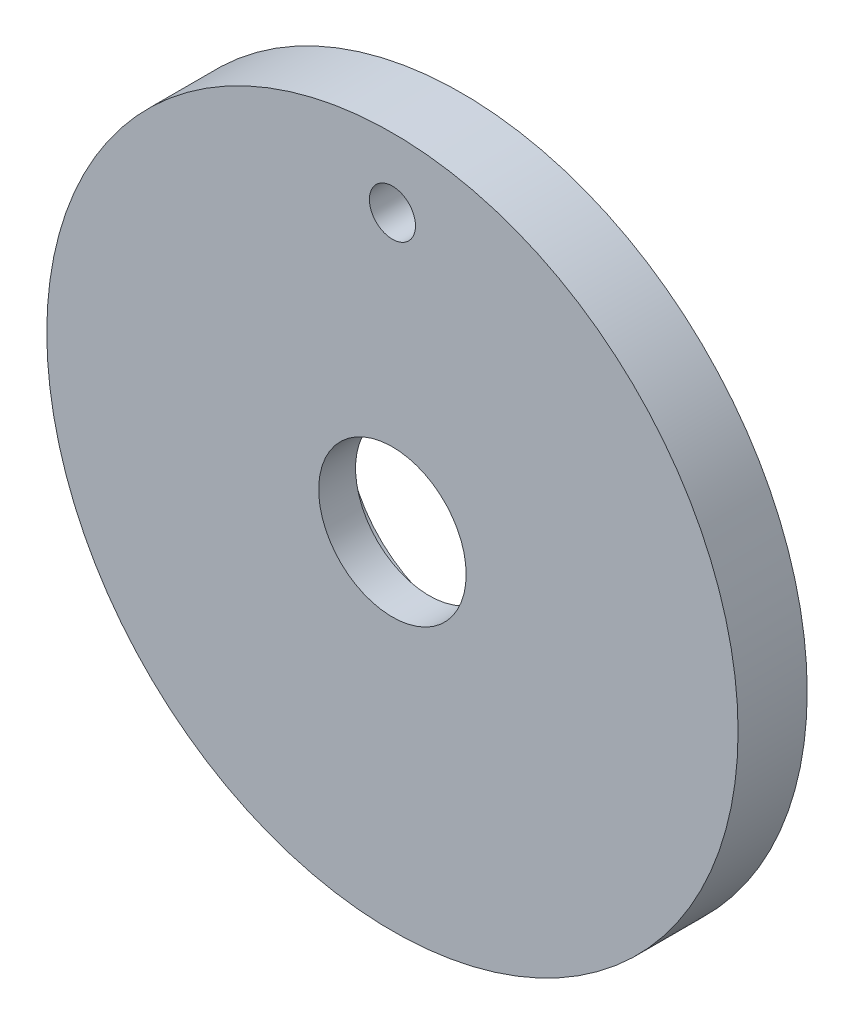
SolidWorks part; units mm, degrees
material "AISI 1045 钢，冷拔"
ref_plane "前视基准面" through (0, 0, 0) normal (0, 0, 1) x (1, 0, 0)
ref_plane "上视基准面" through (0, 0, 0) normal (0, 1, 0) x (1, 0, 0)
ref_plane "右视基准面" through (0, 0, 0) normal (1, 0, 0) x (0, 0, -1)
other "Configuration Table"
sketch "草图1" plane through (0, 0, 0) normal (0, 0, 1) x (1, 0, 0)
  circle A0 centre (0, 0) radius 75
  circle A1 centre (0, 60) radius 5
  circle A2 centre (0, 0) radius 16
  dimension "D1" = 150
  dimension "D2" = 10
  dimension "D4" = 32
  dimension "D3" = 60
extrude "凸台-拉伸1" add sketch "草图1" along normal blind 15
sketch "草图2" plane through (0, 0, 15) normal (0, 0, 1) x (1, 0, 0)
  circle A0 centre (0, 0) radius 25
  dimension "D1" = 50
extrude "切除-拉伸1" cut sketch "草图2" along normal blind 7 from surface at -15 starting at face at (75, 0, 0)
